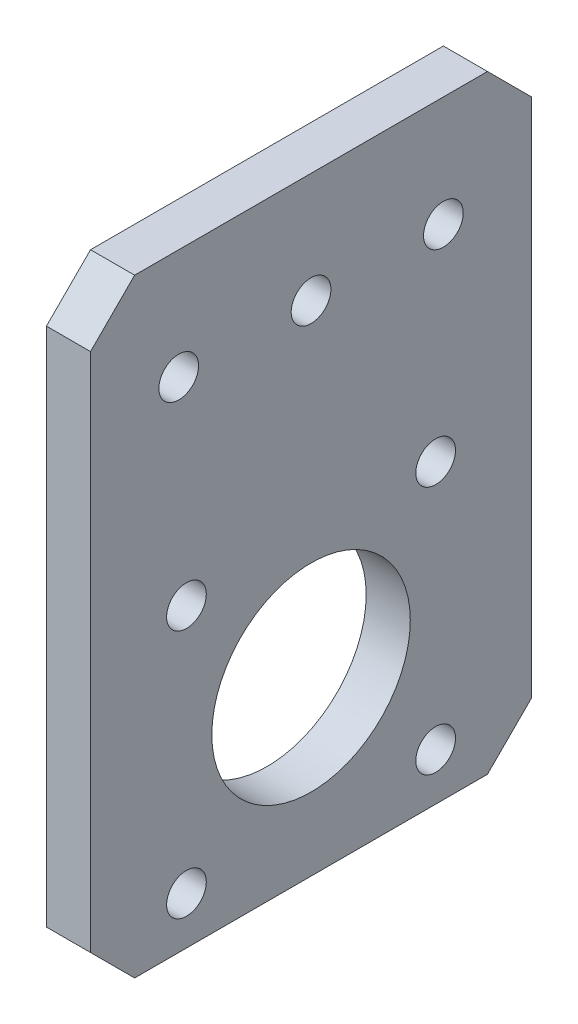
SolidWorks part; units mm, degrees
ref_plane "前视基准面" through (0, 0, 0) normal (0, 0, 1) x (1, 0, 0)
ref_plane "上视基准面" through (0, 0, 0) normal (0, 1, 0) x (1, 0, 0)
ref_plane "右视基准面" through (0, 0, 0) normal (1, 0, 0) x (0, 0, -1)
sketch "草图1" plane through (0, 0, 0) normal (1, 0, 0) x (0, 0, -1)
  line L1 (-50, 69) -> (50, 69)
  line L2 (-50, 69) -> (-50, -69)
  line L3 (-50, -69) -> (50, -69)
  line L4 (50, 69) -> (50, -69)
  line L5 (-50, 69) -> (50, -69) construction
  line L6 (-50, -69) -> (50, 69) construction
  point P0 (0, 0)
  dimension "D1" = 100
  dimension "D2" = 138
extrude "凸台-拉伸1" add sketch "草图1" along normal blind 10
hole_wizard "Ø9.0 (9) 直径孔1" positions "草图2" profile "草图3" hole size "Ø9.0" standard "ISO" end condition through all
sketch "草图2" plane through (10, 0, 0) normal (1, 0, 0) x (0, 0, -1)
  line L0 (0, 41.4164) -> (0, 0) construction
  line L2 (50, 69) -> (-50, 69) construction
  point P0 (-30, 44)
  point P2 (0, 44)
  point P4 (30, 44)
  dimension "D1" = 60
  dimension "D2" = 25
sketch "草图3" plane through (10, 44, 30) normal (0, 1, 0) x (0, 0, -1)
  line L0 (0, 0) -> (0, 10)
  line L1 (0, 10) -> (4.5, 10)
  line L2 (4.5, 10) -> (4.5, 0)
  line L5 (4.5, 0) -> (0, 0)
  line L11 (0, -6.35) -> (0, 107.95) construction
  dimension "通孔孔直径" = 9
  dimension "通孔孔深度" = 10
sketch "草图4" plane through (10, 0, 0) normal (1, 0, 0) x (0, 0, -1)
  line L0 (-50, -69) -> (50, -69) construction
  circle A0 centre (0, -30) radius 22.5
  dimension "D1" = 45
  dimension "D2" = 39
extrude "切除-拉伸1" cut sketch "草图4" against normal blind 10
hole_wizard "Ø9.0 (9) 直径孔2" positions "草图5" profile "草图6" hole size "Ø9.0" standard "ISO" end condition through all
sketch "草图5" plane through (10, 0, 0) normal (1, 0, 0) x (0, 0, -1)
  line L0 (-28.25, -1.75) -> (0, -30) construction
  line L1 (0, -30) -> (0, 0) construction
  point P0 (-28.25, -1.75)
  dimension "D1" = 45
  dimension "D2" = 28.25
sketch "草图6" plane through (10, -1.75, 28.25) normal (0, 1, 0) x (0, 0, -1)
  line L0 (0, 0) -> (0, 10)
  line L1 (0, 10) -> (4.5, 10)
  line L2 (4.5, 10) -> (4.5, 0)
  line L5 (4.5, 0) -> (0, 0)
  line L11 (0, -6.35) -> (0, 107.95) construction
  dimension "通孔孔直径" = 9
  dimension "通孔孔深度" = 10
pattern_circular "阵列(圆周)1" count 4 over 360 about axis through (0, -30, 0) along (1, 0, 0) of "Ø9.0 (9) 直径孔2"
chamfer "倒角1" distance 10 angle 45 4 edges at (5, -69, 50) (5, -69, -50) (5, 69, -50) (5, 69, 50)
